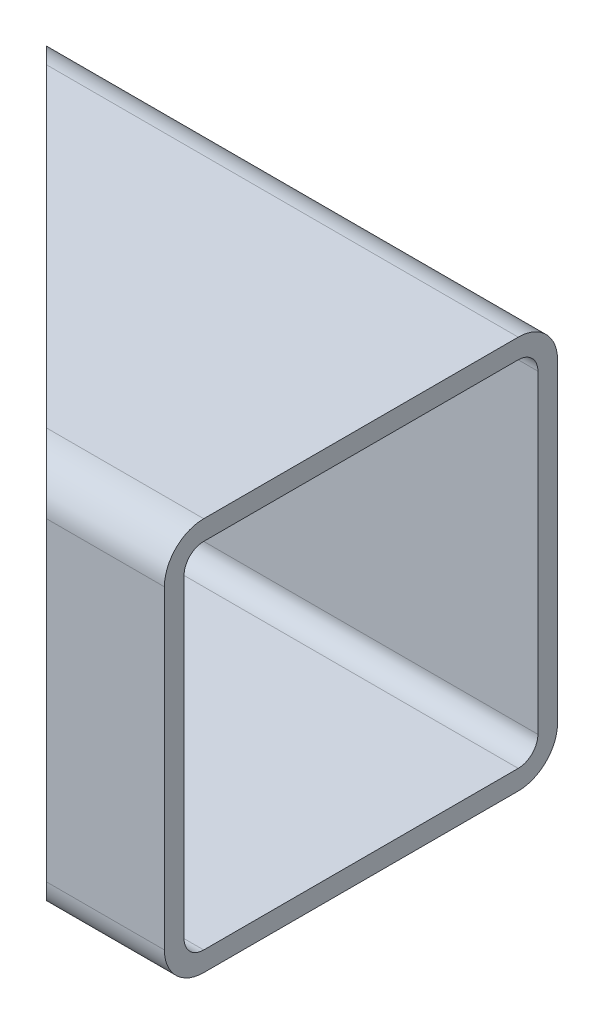
from build123d import *

# Parameters (mm, degrees)
F_100_X_100_X_5_1_DEPTH = 200
CUT_EXTRUDE_1_REACH     = 231.129


with BuildPart() as part:
    # Sketch1 → 方形管 100 X 100 X 5   (1) (new body)
    with BuildSketch(Plane(origin=(0, 0, 0), x_dir=(0, 0, -1), z_dir=(1, 0, 0))):
        with BuildLine():
            Line((-40, -50), (40, -50))
            ThreePointArc((40, -50), (47.071067812, -47.071067812), (50, -40))
            Line((50, -40), (50, 40))
            ThreePointArc((50, 40), (47.071067812, 47.071067812), (40, 50))
            Line((40, 50), (-40, 50))
            ThreePointArc((-40, 50), (-47.071067812, 47.071067812), (-50, 40))
            Line((-50, 40), (-50, -40))
            ThreePointArc((-50, -40), (-47.071067812, -47.071067812), (-40, -50))
        make_face()
        with BuildLine():
            Line((-40, -45), (40, -45))
            ThreePointArc((40, -45), (43.535533906, -43.535533906), (45, -40))
            Line((45, -40), (45, 40))
            ThreePointArc((45, 40), (43.535533906, 43.535533906), (40, 45))
            Line((40, 45), (-40, 45))
            ThreePointArc((-40, 45), (-43.535533906, 43.535533906), (-45, 40))
            Line((-45, 40), (-45, -40))
            ThreePointArc((-45, -40), (-43.535533906, -43.535533906), (-40, -45))
        make_face(mode=Mode.SUBTRACT)
    extrude(amount=F_100_X_100_X_5_1_DEPTH)

    # 切除-拉伸1: up to this face of the body (flat: up to its plane)
    cut_extrude_1_end = Plane(part.part.faces().sort_by_distance((100, -50, 0))[0])
    # 草图2 → 切除-拉伸1 (cut, up to the picked face)
    with BuildSketch(Plane.XZ.offset(-50), mode=Mode.PRIVATE) as cut_extrude_1_sk1:
        Polygon((170, 50), (70, -50), (0, -50), (0, 50), align=None)
    cut_extrude_1_tool1 = split(extrude(cut_extrude_1_sk1.sketch, amount=CUT_EXTRUDE_1_REACH, mode=Mode.PRIVATE), bisect_by=cut_extrude_1_end, keep=Keep.BOTH, mode=Mode.PRIVATE)
    add(cut_extrude_1_tool1.solids().sort_by(Axis((63.472222, 50, 6.944444), (0, -1, 0)))[0], mode=Mode.SUBTRACT)


solid = part.part
